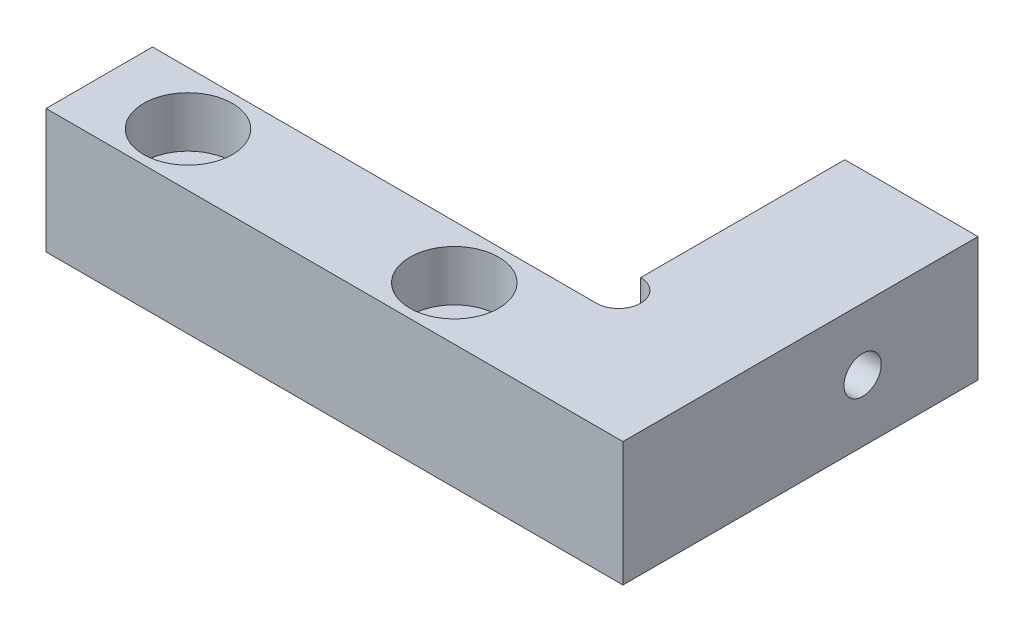
SolidWorks part; units mm, degrees
material "AL6061"
ref_plane "Front Plane" through (0, 0, 0) normal (0, 0, 1) x (1, 0, 0)
ref_plane "Top Plane" through (0, 0, 0) normal (0, 1, 0) x (1, 0, 0)
ref_plane "Right Plane" through (0, 0, 0) normal (1, 0, 0) x (0, 0, -1)
sketch "Sketch1" plane through (0, 0, 0) normal (0, 1, 0) x (1, 0, 0)
  line L9 (-25, -6) -> (25, -6)
  line L10 (-25, -6) -> (-25, 6)
  line L11 (-25, 6) -> (25, 6)
  line L12 (25, -6) -> (25, 6)
  line L13 (-25, -6) -> (25, 6) construction
  line L14 (-25, 6) -> (25, -6) construction
  point P0 (0, 0)
  dimension "D1" = 12
  dimension "D2" = 50
extrude "Boss-Extrude1" add sketch "Sketch1" along normal mid plane 14
hole_wizard "Hole Size (per socket head cap screw type)1" positions "Sketch2" profile "Sketch3" counterbore size "M5" standard "GB" end condition through all
sketch "Sketch2" plane through (0, 7, 0) normal (0, 1, 0) x (1, 0, 0)
  line L0 (0, 0) -> (0, 13.3258) construction
  line L3 (0, 0) -> (-32.8771, 0) construction
  line L4 (-25, 6) -> (-25, -6) construction
  point P13 (-15, 0)
  point P16 (15, 0)
  dimension "D1" = 10
sketch "Sketch3" plane through (15, 7, 0) normal (1, 0, 0) x (0, 0, 1)
  line L0 (0, 0) -> (0, 14)
  line L1 (0, 14) -> (2.75, 14)
  line L3 (2.75, 14) -> (2.75, 5.7)
  line L4 (2.75, 5.7) -> (5, 5.7)
  line L5 (5, 5.7) -> (5, 0)
  line L7 (5, 0) -> (0, 0)
  line L11 (0, -6.35) -> (0, 107.95) construction
  dimension "通孔孔直径" = 5.5
  dimension "通孔孔深度" = 14
  dimension "柱形沉头孔直径" = 10
  dimension "柱形沉头孔深度" = 5.7
sketch "Sketch4" plane through (0, 7, 0) normal (0, 1, 0) x (1, 0, 0)
  line L0 (25, 6) -> (-25, 6) construction
  line L1 (25, -6) -> (40, -6)
  line L2 (25, -6) -> (25, 34)
  line L3 (25, 34) -> (40, 34)
  line L4 (40, -6) -> (40, 34)
  dimension "D1" = 15
  dimension "D2" = 28
extrude "Boss-Extrude2" add sketch "Sketch4" against normal up to surface (14 mm away) up to face at (-15, -7, 2.75)
hole_wizard "M5 Tapped Hole1" positions "Sketch5" profile "Sketch6" tap size "M5" standard "GB" end condition through all
sketch "Sketch5" plane through (40, 0, 0) normal (1, 0, 0) x (0, 0, -1)
  line L0 (0, 0) -> (48.4813, 0) construction
  line L1 (6, 7) -> (6, -7) construction
  point P7 (21, 0)
  dimension "D1" = 15
sketch "Sketch6" plane through (40, 0, -21) normal (0, 1, 0) x (0, 0, -1)
  line L0 (0, 0) -> (0, 65)
  line L1 (0, 65) -> (2.1, 65)
  line L2 (2.1, 65) -> (2.1, 0)
  line L5 (2.1, 0) -> (0, 0)
  line L11 (0, -6.35) -> (0, 107.95) construction
  dimension "通孔螺纹孔钻头直径" = 4.2
  dimension "通孔螺纹孔钻头深度" = 65
cosmetic thread "Hole Thread1" parameters "D2"=5
sketch "Sketch8" plane through (0, 7, 0) normal (0, 1, 0) x (1, 0, 0)
  line L0 (25, 34) -> (25, 6) construction
  circle A0 centre (25, 8.5) radius 2.5
  dimension "D1" = 5
extrude "Cut-Extrude1" cut sketch "Sketch8" against normal through all
